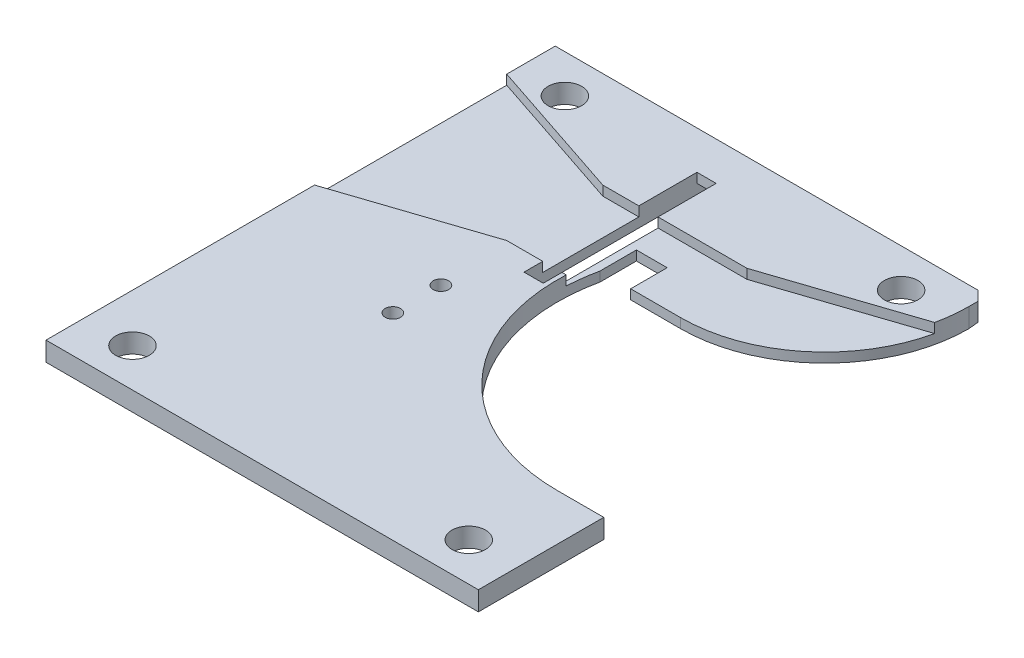
SolidWorks part; units mm, degrees
ref_plane "Front Plane" through (0, 0, 0) normal (0, 0, 1) x (1, 0, 0)
ref_plane "Top Plane" through (0, 0, 0) normal (0, 1, 0) x (1, 0, 0)
ref_plane "Right Plane" through (0, 0, 0) normal (1, 0, 0) x (0, 0, -1)
sketch "Sketch1" plane through (0, 0, 0) normal (0, 1, 0) x (1, 0, 0)
  line L1 (-22.5, 25) -> (22.5, 25)
  line L2 (-22.5, 25) -> (-22.5, -25)
  line L3 (-22.5, -25) -> (22.5, -25)
  line L4 (22.5, 25) -> (22.5, -25)
  line L5 (-22.5, 25) -> (22.5, -25) construction
  line L6 (-22.5, -25) -> (22.5, 25) construction
  point P0 (0, 0)
  dimension "D1" = 45
  dimension "D2" = 50
extrude "Boss-Extrude1" add sketch "Sketch1" along normal blind 2
sketch "Sketch2" plane through (0, 2, 0) normal (0, 1, 0) x (1, 0, 0)
  line L0 (22.5, 25) -> (-22.5, 25) construction
  line L1 (-0.9, 11.85) -> (2.3, 11.85)
  line L2 (-0.9, 11.85) -> (-0.9, 8.05)
  line L3 (-0.9, 8.05) -> (2.3, 8.05)
  line L4 (2.3, 11.85) -> (2.3, 8.05)
  line L5 (-0.9, 11.85) -> (2.3, 8.05) construction
  line L6 (-0.9, 8.05) -> (2.3, 11.85) construction
  line L7 (0.7, 10) -> (0.7, -49990) construction
  line L8 (22.5, -25) -> (22.5, 25) construction
  point P0 (0.7, 9.95)
  dimension "D1" = 15.05
  dimension "D2" = 3.2
  dimension "D3" = 3.8
  dimension "D4" = 21.8
extrude "Cut-Extrude1" cut sketch "Sketch2" against normal through all
sketch "Sketch3" plane through (0, 2, 0) normal (0, 1, 0) x (1, 0, 0)
  line L0 (0.7, 11.85) -> (0.7, 50011.85) construction
  line L1 (2.3, 11.85) -> (-0.9, 11.85) construction
  line L2 (22.5, 25) -> (-22.5, 25) construction
  line L3 (-3.75, 21) -> (-1.75, 21)
  line L4 (-3.75, 21) -> (-3.75, 3)
  line L5 (-3.75, 3) -> (-1.75, 3)
  line L6 (-1.75, 21) -> (-1.75, 3)
  line L7 (-3.75, 21) -> (-1.75, 3) construction
  line L8 (-3.75, 3) -> (-1.75, 21) construction
  point P4 (0.7, 11.85)
  point P5 (-2.75, 12)
  dimension "D1" = 3.45
  dimension "D2" = 2
  dimension "D3" = 18
  dimension "D4" = 22
extrude "Cut-Extrude2" cut sketch "Sketch3" against normal through all
sketch "Sketch4" plane through (0, 0, 0) normal (0, -1, 0) x (1, 0, 0)
  line L0 (22.5, -25) -> (-22.5, -25) construction
  line L1 (-3.75, -21) -> (-1.75, -21)
  line L2 (-3.75, -21) -> (-3.75, -25)
  line L3 (-3.75, -25) -> (-1.75, -25)
  line L4 (-1.75, -21) -> (-1.75, -25)
  line L5 (-1.75, -3) -> (-1.75, -21) construction
extrude "Cut-Extrude3" cut sketch "Sketch4" against normal blind 1
sketch "Sketch5" plane through (0, 2, 0) normal (0, 1, 0) x (1, 0, 0)
  line L0 (4.8, 9.95) -> (50004.8, 9.95) construction
  line L1 (2.3, 8.05) -> (2.3, 11.85) construction
  line L2 (-1006.6, 8.05) -> (-0.9, 8.05) construction
  line L5 (46.771, 8.05) -> (50004.8, 8.05) construction
  line L6 (-0.9, 8.05) -> (26.4614, 8.05)
  line L7 (26.4614, 8.05) -> (36.2484, 8.05)
  line L8 (-0.0742, 8.05) -> (36.2484, 8.05) construction
  line L9 (18.5, 4.05) -> (50018.5, 4.05) construction
  arc A1 (-0.9, 8.05) -> (36.2484, 8.05) centre (17.6742, 4.05) ccw
  point P4 (2.3, 9.95)
  dimension "D4" = 38
extrude "Cut-Extrude4" cut sketch "Sketch5" against normal blind 3
sketch "Sketch6" plane through (0, 2, 0) normal (0, 1, 0) x (1, 0, 0)
  line L0 (2.3, 9.95) -> (50002.3, 9.95) construction
  line L1 (2.3, 8.05) -> (2.3, 11.85) construction
  line L2 (-0.9, 11.85) -> (-0.9, 8.05) construction
  line L3 (-24.3, 4.95) -> (22.5, 4.95)
  line L4 (-24.3, 4.95) -> (-24.3, 14.95)
  line L5 (-24.3, 14.95) -> (22.5, 14.95)
  line L6 (22.5, 4.95) -> (22.5, 14.95)
  line L7 (-24.3, 4.95) -> (22.5, 14.95) construction
  line L8 (-24.3, 14.95) -> (22.5, 4.95) construction
  line L9 (22.5, 8.05) -> (22.5, 25) construction
  point P4 (2.3, 9.95)
  point P5 (-0.9, 9.95)
  dimension "D1" = 10
extrude "Cut-Extrude5" cut sketch "Sketch6" against normal blind 1
chamfer "Chamfer1" distance 15 distance2 5 2 edges at (-22.5, 1.5, -4.95) (-22.5, 1.5, -14.95)
chamfer "Chamfer2" distance 5 distance2 15 1 edges at (22.5, 1.5, -14.95)
sketch "Sketch8" plane through (0, 0, 25) normal (0, 0, 1) x (1, 0, 0)
  line L1 (-22.5, 2) -> (22.5, 2)
  line L2 (-22.5, 2) -> (-22.5, 0)
  line L3 (-22.5, 0) -> (22.5, 0)
  line L4 (22.5, 2) -> (22.5, 0)
extrude "Boss-Extrude2" add sketch "Sketch8" along normal blind 3
sketch "Sketch7" plane through (0, 2, 0) normal (0, 1, 0) x (1, 0, 0)
  line L0 (0, 25) -> (0, -49975) construction
  line L1 (22.5, 25) -> (-22.5, 25) construction
  circle A0 centre (-17.5, 21) radius 1.75
  circle A1 centre (17.5, 21) radius 1.75
  circle A2 centre (17.5, -24) radius 1.75
  circle A3 centre (-17.5, -24) radius 1.75
  point P4 (0, 25)
  dimension "D1" = 3.5
  dimension "D2" = 35
  dimension "D3" = 45
  dimension "D4" = 4
extrude "Cut-Extrude6" cut sketch "Sketch7" against normal through all
fillet "Fillet2" radius 15 1 edges at (22.5, 0.5, -8.05)
chamfer "Chamfer4" distance 2 distance2 0.2 2 edges at (10.375, 0, -25) (-13.125, 0, -25)
sketch "Sketch10" plane through (0, 2, 0) normal (0, 1, 0) x (1, 0, 0)
  line L0 (22.5, -28) -> (22.5, -14.3269) construction
  line L1 (17.6742, -14.95) -> (22.5, -14.95)
  line L2 (17.6742, -14.95) -> (17.6742, -11.9986)
  line L3 (17.6742, -11.9986) -> (22.5, -11.9986)
  line L4 (22.5, -14.95) -> (22.5, -11.9986)
  line L5 (17.6742, -14.95) -> (17.6742, -14.0499) construction
  arc A0 (-0.9, 8.05) -> (22.5, -14.3269) centre (17.6742, 4.05) ccw construction
extrude "Cut-Extrude7" cut sketch "Sketch10" against normal through all
chamfer "Chamfer5" distance 1 angle 45 1 edges at (22.5, 1.1, -25)
hole_wizard "M2 Tapped Hole1" positions "Sketch12" profile "Sketch11" tap size "M2" standard "Gb"
sketch "Sketch12" plane through (0, 2, 0) normal (0, 1, 0) x (1, 0, 0)
  point P0 (-6.9, -7.5)
  point P3 (-6.9, -2.5)
sketch "Sketch11" plane through (-6.9, 2, 7.5) normal (1, 0, 0) x (0, 0, 1)
  line L0 (0, 0) -> (0, 5.6807)
  line L1 (0, 5.6807) -> (0.8, 5.2)
  line L2 (0.8, 5.2) -> (0.8, 0)
  line L5 (0.8, 0) -> (0, 0)
  line L10 (0, 5.6807) -> (-0.8, 5.2) construction
  line L11 (0, -6.35) -> (0, 107.95) construction
  dimension "螺纹孔钻头直径" = 1.6
  dimension "螺纹孔钻头深度" = 5.2
  dimension "导头角度" = 118
cosmetic thread "Cosmetic Thread1" parameters "D1"=2, "D2"=2
cosmetic thread "Cosmetic Thread2" parameters "D1"=2, "D2"=2
